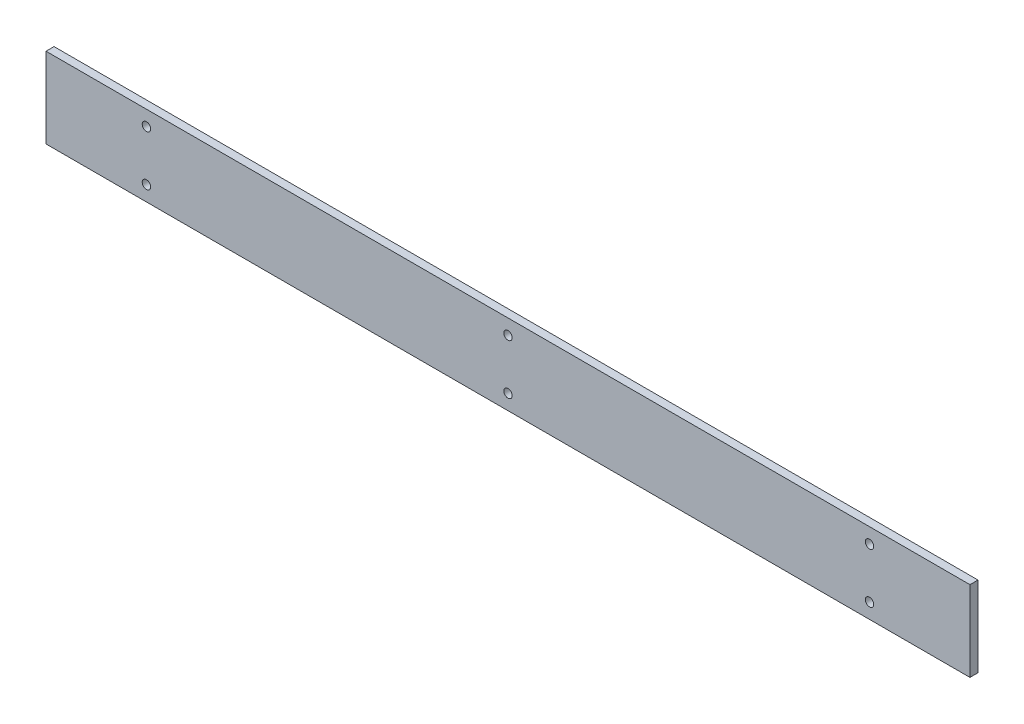
from build123d import *

# Parameters (mm, degrees)
SKETCH_1_W             = 460
SKETCH_1_H             = 40
EXTRUDE_1_DEPTH        = 2
HOLE_WIZARD_M5_1_D     = 4.2
HOLE_WIZARD_M5_1_DEPTH = 14
HOLE_WIZARD_M5_1_TIP   = 1.2618073


with BuildPart() as part:
    # 草图1 → 凸台-拉伸1 (new, symmetric)
    with BuildSketch(Plane.XY):
        Rectangle(SKETCH_1_W, SKETCH_1_H)
    extrude(amount=EXTRUDE_1_DEPTH, both=True)

    # M5 螺纹孔1
    with Locations(Plane.XY.offset(2)):
        with Locations((-180, 12.5), (-180, -12.5), (0, 12.5), (0, -12.5), (180, 12.5), (180, -12.5)):
            Hole(HOLE_WIZARD_M5_1_D / 2, depth=HOLE_WIZARD_M5_1_DEPTH)
            with Locations((0, 0, -(HOLE_WIZARD_M5_1_DEPTH + HOLE_WIZARD_M5_1_TIP / 2))):  # 118° drill point
                Cone(0, HOLE_WIZARD_M5_1_D / 2, HOLE_WIZARD_M5_1_TIP, mode=Mode.SUBTRACT)


solid = part.part
